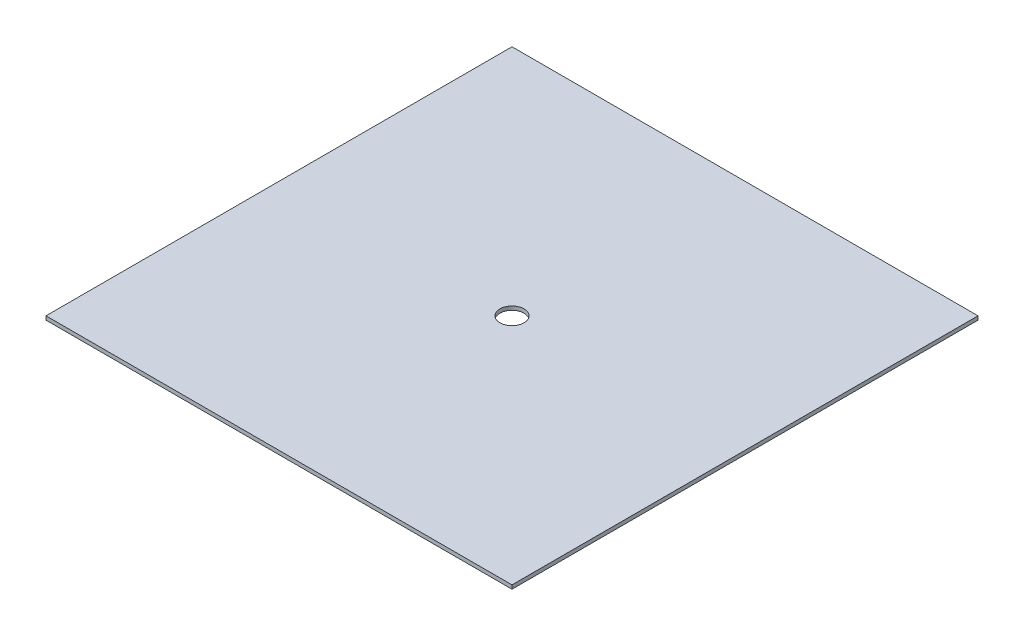
from build123d import *

# Parameters (mm, degrees)
SKETCH1_W           = 98.4
SKETCH1_H           = 98.4
SKETCH1_R           = 2.55
BOSS_EXTRUDE1_DEPTH = 0.8


with BuildPart() as part:
    # Sketch1 → Boss-Extrude1 (new body)
    with BuildSketch(Plane(origin=(0, 0, 0), x_dir=(1, 0, 0), z_dir=(0, 1, 0))):
        Rectangle(SKETCH1_W, SKETCH1_H)
        with Locations(Location((0, 0, 0), (0, 0, 270))):
            Circle(SKETCH1_R, mode=Mode.SUBTRACT)
    extrude(amount=BOSS_EXTRUDE1_DEPTH)


solid = part.part
